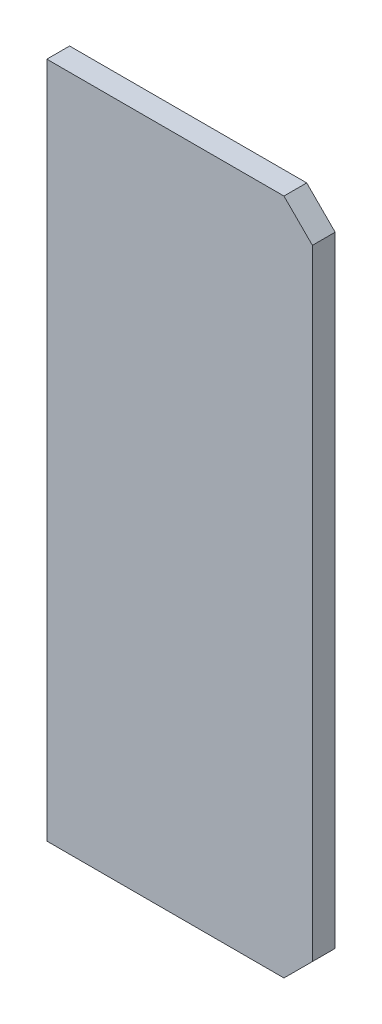
from build123d import *

# Parameters (mm, degrees)
SKETCH1_W           = 140
SKETCH1_H           = 357
BOSS_EXTRUDE1_DEPTH = 12
CHAMFER2_SIZE       = 15


with BuildPart() as part:
    # Sketch1 → Boss-Extrude1 (new body)
    with BuildSketch(Plane.XY):
        with Locations((70, 178.5)):
            Rectangle(SKETCH1_W, SKETCH1_H)
    extrude(amount=BOSS_EXTRUDE1_DEPTH)

    # Chamfer2
    chamfer2_edges = [part.edges().sort_by_distance(p)[0] for p in [
        (140, 357, 6),
        (140, 0, 6),
    ]]
    chamfer(chamfer2_edges, length=CHAMFER2_SIZE)


solid = part.part
